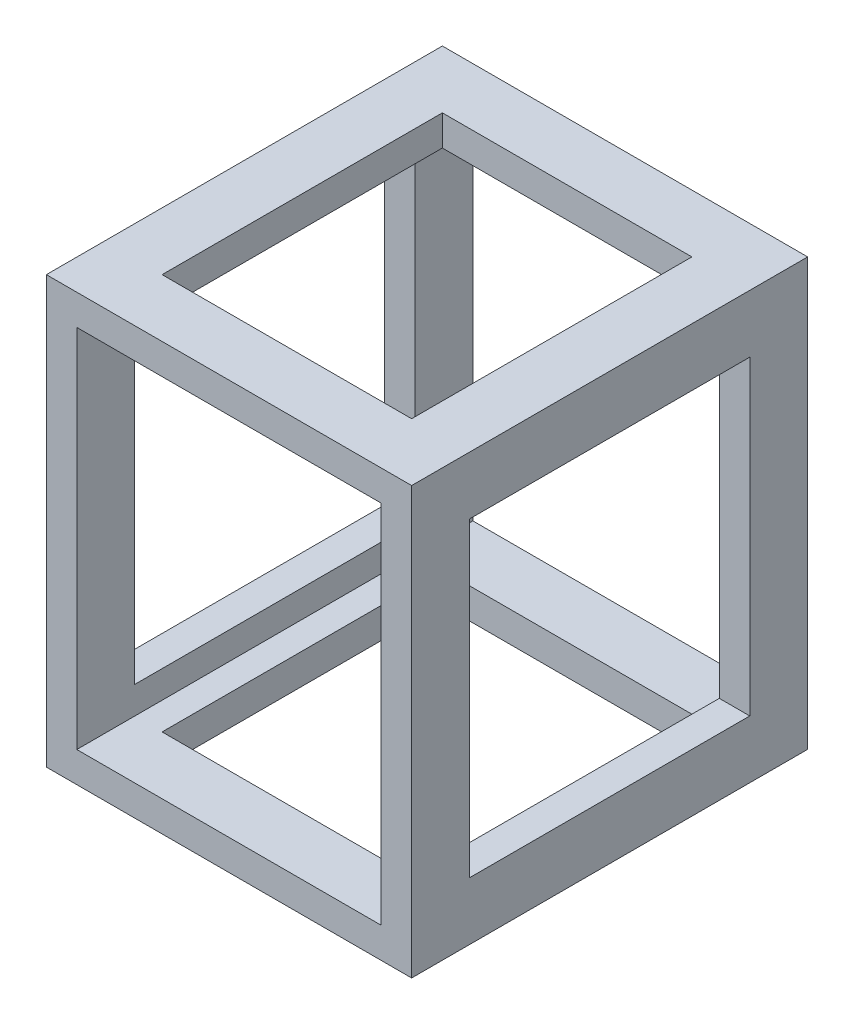
from build123d import *

# Parameters (mm, degrees)
SKETCH1_W           = 119.911519959
SKETCH1_H           = 140
SKETCH1_W_2         = 99.911519959
SKETCH1_H_2         = 120
BOSS_EXTRUDE1_DEPTH = 130
SKETCH2_W           = 81.911519959
SKETCH2_H           = 92
CUT_EXTRUDE1_DEPTH  = 258
SKETCH3_W           = 92
SKETCH3_H           = 102
CUT_EXTRUDE2_DEPTH  = 258


with BuildPart() as part:
    # Sketch1 → Boss-Extrude1 (new body)
    with BuildSketch(Plane.XY):
        with Locations((-10.04424002, 160)):
            Rectangle(SKETCH1_W, SKETCH1_H)
        with Locations((-10.044240021, 160)):
            Rectangle(SKETCH1_W_2, SKETCH1_H_2, mode=Mode.SUBTRACT)
    extrude(amount=-BOSS_EXTRUDE1_DEPTH)

    # Sketch2 → Cut-Extrude1 (cut)
    with BuildSketch(Plane.XZ.offset(-90)):
        with Locations((-10.04424002, -65)):
            Rectangle(SKETCH2_W, SKETCH2_H)
    extrude(amount=-CUT_EXTRUDE1_DEPTH, mode=Mode.SUBTRACT)

    # Sketch3 → Cut-Extrude2 (cut)
    with BuildSketch(Plane.ZY.offset(70)):
        with Locations((-65, 160)):
            Rectangle(SKETCH3_W, SKETCH3_H)
    extrude(amount=-CUT_EXTRUDE2_DEPTH, mode=Mode.SUBTRACT)


solid = part.part
